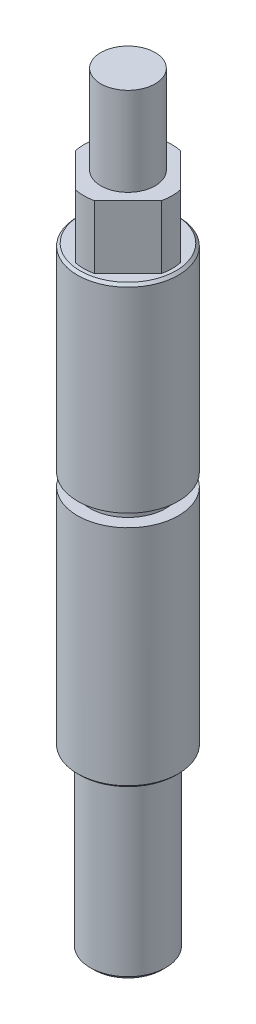
from build123d import *

# Parameters (mm, degrees)
BOSS_EXTRUDE1_START = 13.904652831
SKETCH2_R           = 3
BOSS_EXTRUDE1_DEPTH = 13.904652831
BOSS_EXTRUDE2_DEPTH = 5
SKETCH4_R           = 2.15
BOSS_EXTRUDE3_DEPTH = 7
CHAMFER1_SIZE       = 0.2
CHAMFER2_SIZE       = 0.3


with BuildPart() as part:
    # Sketch1 → Revolve1 (revolve)
    with BuildSketch(Plane(origin=(0, 0, 0), x_dir=(-1, 0, 0), z_dir=(0, 0, -1)), mode=Mode.PRIVATE) as revolve1_sk:
        Polygon((-4, -29.495347169), (0, -29.495347169), (0, 5.1), (-4, 5.1), (-4, -10.6), (-3, -10.6), (-3, -11.6), (-4, -11.6), align=None)
    revolve(revolve1_sk.sketch.rotate(Axis((0, -29.495347169, 0), (0, 1, 0)), 270), axis=Axis((0, -29.495347169, 0), (0, 1, 0)))

    # Sketch2 → Boss-Extrude1 (add)
    with BuildSketch(Plane.XZ.offset(29.495347169).offset(BOSS_EXTRUDE1_START)):
        with Locations(Location((0, 0, 0), (0, 0, 90))):
            Circle(SKETCH2_R)
    extrude(amount=-BOSS_EXTRUDE1_DEPTH)

    # Sketch3 → Boss-Extrude2 (add)
    with BuildSketch(Plane(origin=(0, 5.1, 0), x_dir=(-1, 0, 0), z_dir=(0, 1, 0))):
        with BuildLine():
            Line((3.417793986, -0.754111574), (0.754142944, -3.417787065))
            ThreePointArc((0.754142944, -3.417787065), (1.6062e-05, -3.5), (-0.754111574, -3.417793986))
            Line((-0.754111574, -3.417793986), (-3.417787065, -0.754142944))
            ThreePointArc((-3.417787065, -0.754142944), (-3.5, -1.6062e-05), (-3.417793986, 0.754111574))
            Line((-3.417793986, 0.754111574), (-0.754142944, 3.417787065))
            ThreePointArc((-0.754142944, 3.417787065), (0, 3.5), (0.754142944, 3.417787065))
            Line((0.754142944, 3.417787065), (3.417787065, 0.754142944))
            ThreePointArc((3.417787065, 0.754142944), (3.5, 1.6062e-05), (3.417793986, -0.754111574))
        make_face()
    extrude(amount=BOSS_EXTRUDE2_DEPTH)

    # Sketch4 → Boss-Extrude3 (add)
    with BuildSketch(Plane(origin=(0, 10.1, 0), x_dir=(-1, 0, 0), z_dir=(0, 1, 0))):
        with Locations(Location((0, 0, 0), (0, 0, 90))):
            Circle(SKETCH4_R)
    extrude(amount=BOSS_EXTRUDE3_DEPTH)

    # Chamfer1
    chamfer1_edges = [part.edges().sort_by_distance(p)[0] for p in [
        (0, -29.495347169, -4),
        (0, 5.1, -4),
    ]]
    chamfer(chamfer1_edges, length=CHAMFER1_SIZE)

    # Chamfer2
    chamfer2_edges = [part.edges().sort_by_distance(p)[0] for p in [
        (0, -43.4, -3),
    ]]
    chamfer(chamfer2_edges, length=CHAMFER2_SIZE)


solid = part.part
